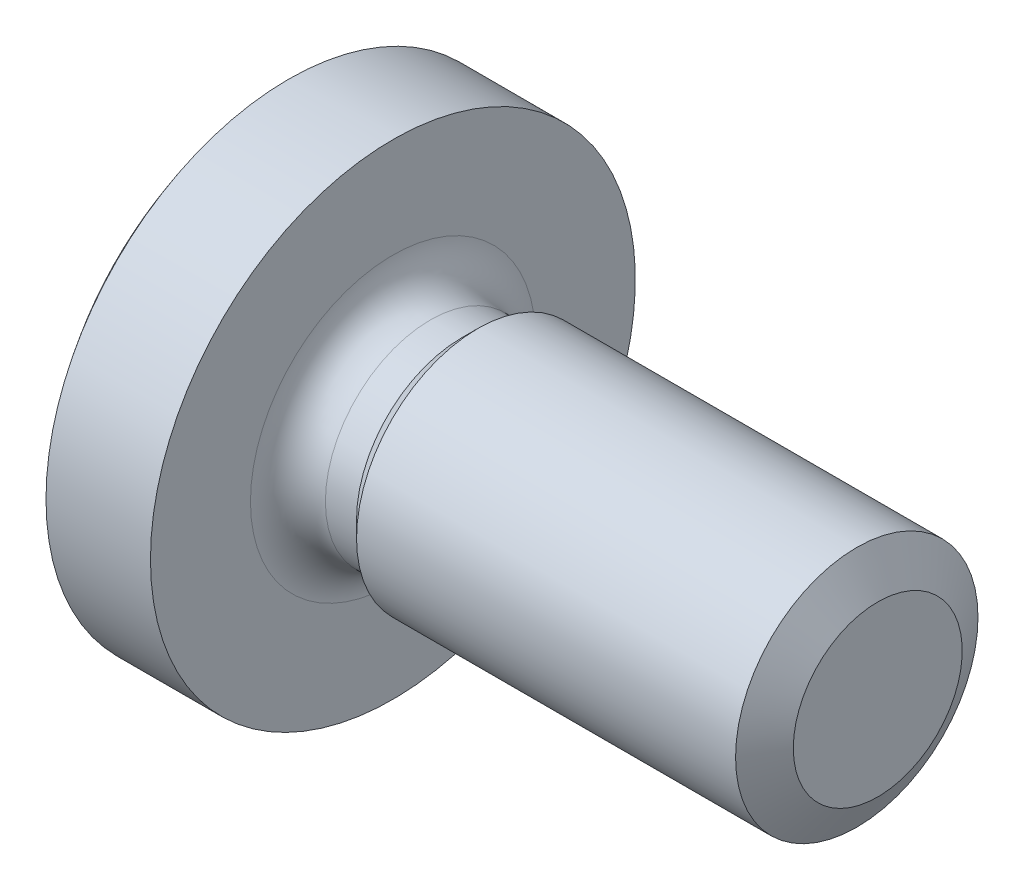
from build123d import *


with BuildPart() as part:
    # Sketch2 → Base-Revolve (revolve)
    with BuildSketch(Plane.XY, mode=Mode.PRIVATE) as base_revolve_sk:
        with BuildLine():
            Line((0, 0), (11.1, 0))
            Line((11.1, 0), (11.1, 2))
            Line((11.1, 2), (4.5, 2))
            Line((4.5, 2), (4.232, 1.732))
            Line((4.232, 1.732), (3.718, 1.732))
            ThreePointArc((3.718, 1.732), (3.281008009, 1.913008009), (3.1, 2.35))
            Line((3.1, 2.35), (3.1, 4))
            Line((3.1, 4), (1.376524617, 4))
            ThreePointArc((1.376524617, 4), (0.353757652, 2.115113473), (0, 0))
        make_face()
    revolve(base_revolve_sk.sketch.rotate(Axis((-1.331757704, 0, 0), (1, 0, 0)), 90), axis=Axis((-1.331757704, 0, 0), (1, 0, 0)))

    # Sketch3 → Cut-Revolve1 (revolve, cut)
    with BuildSketch(Plane.XY, mode=Mode.PRIVATE) as cut_revolve1_sk:
        Polygon((10.753791204, 2), (11.453791204, 2), (11.1, 1.3938), align=None)
    revolve(cut_revolve1_sk.sketch.rotate(Axis((-0.242766179, 0, 0), (1, 0, 0)), 90), axis=Axis((-0.242766179, 0, 0), (1, 0, 0)), mode=Mode.SUBTRACT)

    # Sketch5 → Cut-Loft1 section 0
    with BuildSketch(Plane(origin=(0, 0, 0), x_dir=(0, 0, -1), z_dir=(1, 0, 0)), mode=Mode.PRIVATE) as cut_loft1_s0:
        with BuildLine():
            Line((0.35, 2.2), (-0.35, 2.2))
            Line((-0.35, 2.2), (-0.35, -2.2))
            Line((-0.35, -2.2), (0.35, -2.2))
            Line((0.35, -2.2), (0.35, 2.2))
        make_face()
    cut_loft1 = loft([Vertex(2.4, 0, 0), cut_loft1_s0.sketch], mode=Mode.SUBTRACT)

    # Mirror1: Cut-Loft1 across plane
    add(cut_loft1.mirror(Plane(origin=(0, 0, 0), x_dir=(0, 0.7071067811865462, 0.7071067811865488), z_dir=(0, -0.7071067811865488, 0.7071067811865462))), mode=Mode.SUBTRACT)


solid = part.part
